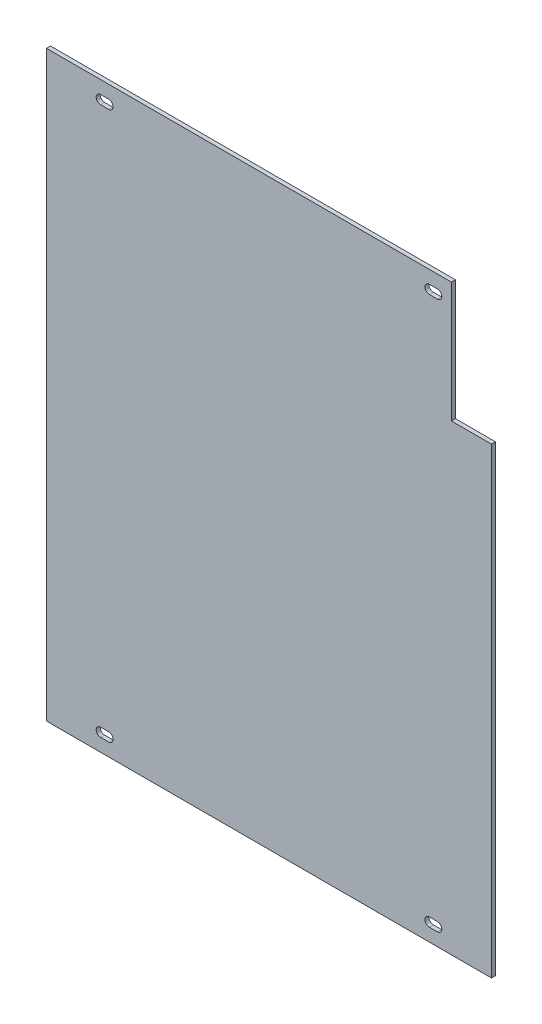
SolidWorks part; units mm, degrees
ref_plane "前视基准面" through (0, 0, 0) normal (0, 0, 1) x (1, 0, 0)
ref_plane "上视基准面" through (0, 0, 0) normal (0, 1, 0) x (1, 0, 0)
ref_plane "右视基准面" through (0, 0, 0) normal (1, 0, 0) x (0, 0, -1)
sketch "草图1" plane through (0, 0, 0) normal (0, 0, 1) x (1, 0, 0)
  line L1 (166.5, -218) -> (-166.5, -218)
  line L2 (166.5, -218) -> (166.5, 218)
  line L3 (166.5, 218) -> (-166.5, 218)
  line L4 (-166.5, -218) -> (-166.5, 218)
  line L5 (166.5, -218) -> (-166.5, 218) construction
  line L6 (166.5, 218) -> (-166.5, -218) construction
  point P0 (0, 0)
  dimension "D1" = 333
  dimension "D2" = 436
extrude "凸台-拉伸1" add sketch "草图1" along normal blind 3
sketch "草图3" plane through (0, 0, 0) normal (0, 0, -1) x (-1, 0, 0)
  line L1 (-136.5, 128) -> (-166.5, 128)
  line L2 (-136.5, 128) -> (-136.5, 218)
  line L3 (-136.5, 218) -> (-166.5, 218)
  line L4 (-166.5, 128) -> (-166.5, 218)
  line L5 (-136.5, 128) -> (-166.5, 218) construction
  line L6 (-136.5, 218) -> (-166.5, 128) construction
  point P0 (-151.5, 173)
  dimension "D1" = 90
  dimension "D2" = 30
extrude "切除-拉伸2" cut sketch "草图3" against normal blind 10
sketch "草图4" plane through (0, 0, 3) normal (0, 0, 1) x (1, 0, 0)
  line L7 (120, -205) -> (-120, -205) construction
  line L8 (120, -205) -> (120, 205) construction
  line L9 (120, 205) -> (-120, 205) construction
  line L10 (-120, -205) -> (-120, 205) construction
  line L11 (120, -205) -> (-120, 205) construction
  line L12 (120, 205) -> (-120, -205) construction
  line L25 (-120, 205) -> (-126, 205) construction
  line L26 (-120, 201.7) -> (-126, 201.7)
  line L27 (-120, 208.3) -> (-126, 208.3)
  line L28 (120, 205) -> (126, 205) construction
  line L29 (120, 208.3) -> (126, 208.3)
  line L30 (120, 201.7) -> (126, 201.7)
  line L35 (120, -205) -> (126, -205) construction
  line L43 (120, -201.7) -> (126, -201.7)
  line L44 (120, -208.3) -> (126, -208.3)
  line L45 (-120, -205) -> (-126, -205) construction
  line L46 (-120, -208.3) -> (-126, -208.3)
  line L47 (-120, -201.7) -> (-126, -201.7)
  arc A0 (-120, 201.7) -> (-120, 208.3) centre (-120, 205) ccw
  arc A1 (-126, 208.3) -> (-126, 201.7) centre (-126, 205) ccw
  arc A2 (120, 208.3) -> (120, 201.7) centre (120, 205) ccw
  arc A3 (126, 201.7) -> (126, 208.3) centre (126, 205) ccw
  arc A4 (120, -201.7) -> (120, -208.3) centre (120, -205) ccw
  arc A5 (126, -208.3) -> (126, -201.7) centre (126, -205) ccw
  arc A6 (-120, -208.3) -> (-120, -201.7) centre (-120, -205) ccw
  arc A7 (-126, -201.7) -> (-126, -208.3) centre (-126, -205) ccw
  point P0 (0, 0)
  point P5 (-123, 205)
  point P11 (123, 205)
  point P17 (123, -205)
  point P24 (-123, -205)
  dimension "D3" = 3.3
  dimension "D1" = 410
  dimension "D2" = 240
  dimension "D4" = 6
extrude "切除-拉伸3" cut sketch "草图4" against normal blind 10
